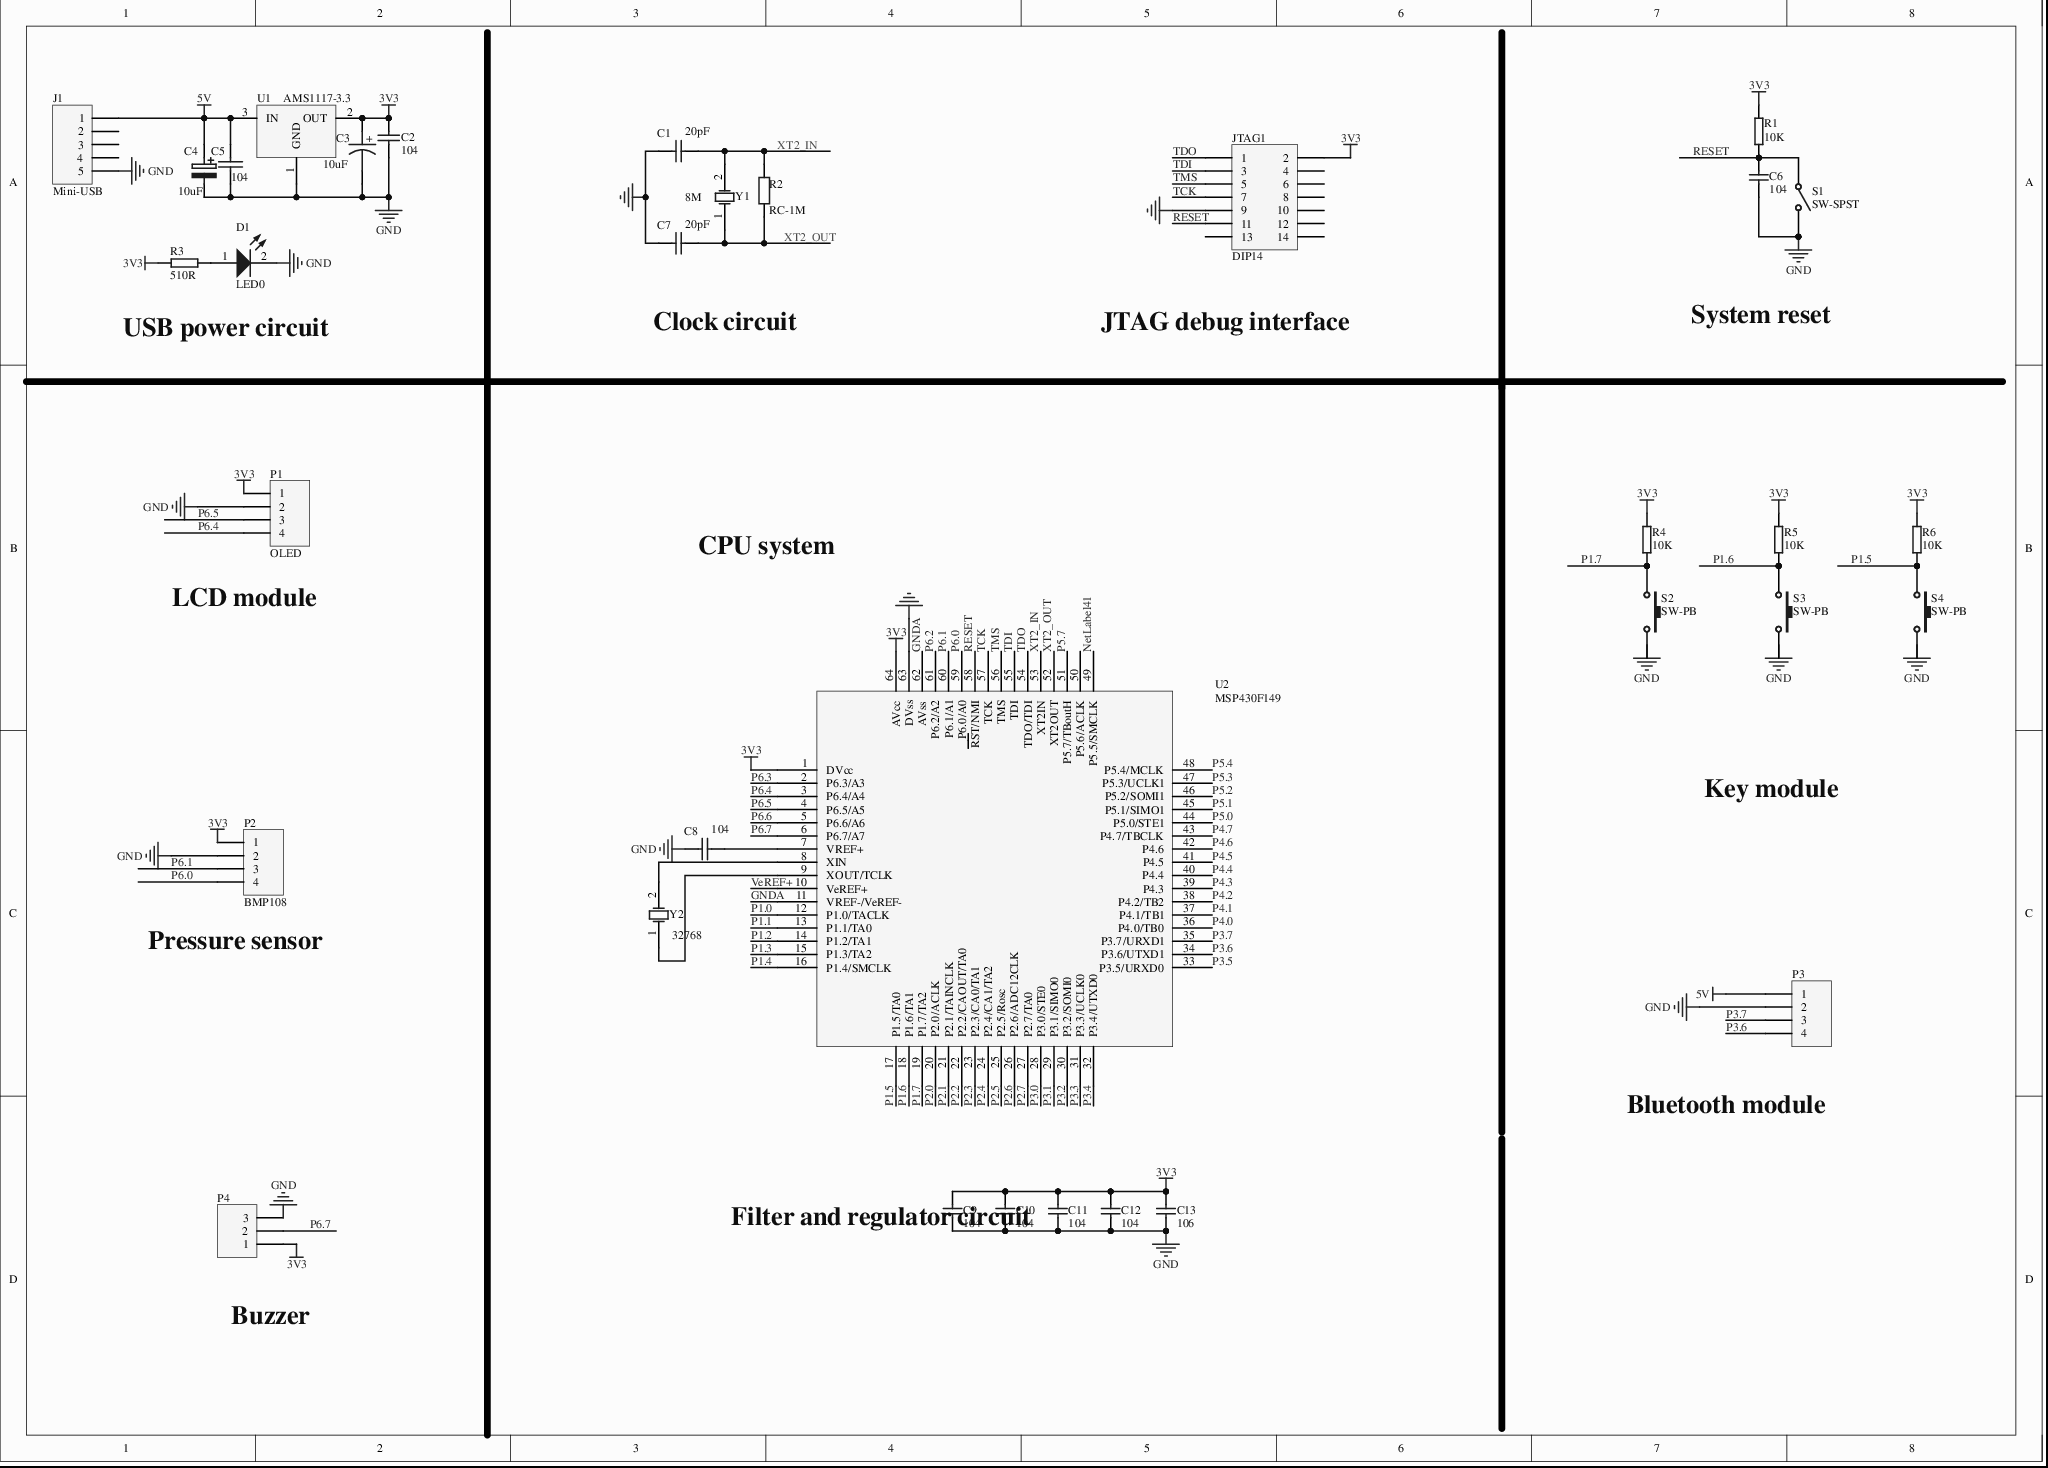
[diagram p0: MISC82806-6.SchDoc]
# Altium project MISC82806-6.PrjPcb
1 sheet, 34 parts. Net scope: global (net labels, ports and power ports of the same name join across sheets).
Board file: MISC82806.PcbDoc

## Sheet MISC82806-6.SchDoc
size A3

### Parts
C1  value 20pF  [0805C]  (hidden comment: S0805-20P)
C2  104  [0603C]
C3  10uF  [贴片电容]
C4  10uF  [0805C]
C5  104  [0603C]
C6  104  [0603C]
C7  value 20pF  [0805C]  (hidden comment: S0805-20P)
C8  value 104  [0805C]  (hidden comment: S0805-20P)
C9  104  [0603C]
C10  104  [0603C]
C11  104  [0603C]
C12  104  [0603C]
C13  106  [0805C]
D1  LED0  [LED0603-RD]
J1  Mini-USB  [USB-MINI-A]
JTAG1  DIP14  [HDR2X7]
P1  OLED  [HDR1X4H]
P2  BMP108  [HDR1X4H]
P3  Bluetooth module  [HDR1X4]  (value not drawn)
P4  Buzzer  [HDR1X3]  (value not drawn)
R1  10K  [0603R]
R2  RC-1M  [0805R]
R3  510R  [0603R]
R4  10K  [0603R]
R5  10K  [0603R]
R6  10K  [0603R]
S1  SW-SPST  [SPST-2]
S2  SW-PB  [SPST-2]
S3  SW-PB  [SPST-2]
S4  SW-PB  [SPST-2]
U1  AMS1117-3.3  [AMS1117-3.3]
U2  MSP430F149  [MSP430F149]
Y1  8M  [XTAL-SMD-NX3215SA-32.768K-STD-MUS-2]
Y2  32768  [XTAL-SMD-NX3215SA-32.768K-STD-MUS-2]

### Nets
3V3: C2.1 C3.1 C9.1 C10.1 C11.1 C12.1 C13.1 JTAG1.2 P1.1 P2.1 P4.1 R1.2 R3.2 R4.2 R5.2 R6.2 U1.2(OUT) U2.1(DVcc) U2.64(AVcc)
5V: C4.1 C5.1 J1.1 P3.1 U1.3(IN)
GND: C1.1 C2.2 C3.2 C4.2 C5.2 C6.2 C7.1 C8.1 C9.2 C10.2 C11.2 C12.2 C13.2 D1.2(K) J1.5 JTAG1.9 P1.2 P2.2 P3.2 P4.3 S1.2(NO) U1.1(GND) U2.63(DVss)
GNDA: U2.11(VREF-/VeREF-) U2.62(AVss)
NetLabel41: U2.49(P5.5/SMCLK)
P1.0: U2.12(P1.0/TACLK)
P1.1: U2.13(P1.1/TA0)
P1.2: U2.14(P1.2/TA1)
P1.3: U2.15(P1.3/TA2)
P1.4: U2.16(P1.4/SMCLK)
P1.5: R6.1 S4.1 U2.17(P1.5/TA0)
P1.6: R5.1 S3.1 U2.18(P1.6/TA1)
P1.7: R4.1 S2.1 U2.19(P1.7/TA2)
P2.0: U2.20(P2.0/ACLK)
P2.1: U2.21(P2.1/TAINCLK)
P2.2: U2.22(P2.2/CAOUT/TA0)
P2.3: U2.23(P2.3/CA0/TA1)
P2.4: U2.24(P2.4/CA1/TA2)
P2.5: U2.25(P2.5/Rosc)
P2.6: U2.26(P2.6/ADC12CLK)
P2.7: U2.27(P2.7/TA0)
P3.0: U2.28(P3.0/STE0)
P3.1: U2.29(P3.1/SIMO0)
P3.2: U2.30(P3.2/SOMI0)
P3.3: U2.31(P3.3/UCLK0)
P3.4: U2.32(P3.4/UTXD0)
P3.5: U2.33(P3.5/URXD0)
P3.6: P3.4 U2.34(P3.6/UTXD1)
P3.7: P3.3 U2.35(P3.7/URXD1)
P4.0: U2.36(P4.0/TB0)
P4.1: U2.37(P4.1/TB1)
P4.2: U2.38(P4.2/TB2)
P4.3: U2.39(P4.3)
P4.4: U2.40(P4.4)
P4.5: U2.41(P4.5)
P4.6: U2.42(P4.6)
P4.7: U2.43(P4.7/TBCLK)
P5.0: U2.44(P5.0/STE1)
P5.1: U2.45(P5.1/SIMO1)
P5.2: U2.46(P5.2/SOMI1)
P5.3: U2.47(P5.3/UCLK1)
P5.4: U2.48(P5.4/MCLK)
P5.7: U2.51(P5.7/TBoutH)
P6.0: P2.4 U2.59(P6.0/A0)
P6.1: P2.3 U2.60(P6.1/A1)
P6.2: U2.61(P6.2/A2)
P6.3: U2.2(P6.3/A3)
P6.4: P1.4 U2.3(P6.4/A4)
P6.5: P1.3 U2.4(P6.5/A5)
P6.6: U2.5(P6.6/A6)
P6.7: P4.2 U2.6(P6.7/A7)
RESET: C6.1 JTAG1.11 R1.1 S1.1(COMMON) U2.58(~{RS}T/NMI)
TCK: JTAG1.7 U2.57(TCK)
TDI: JTAG1.3 U2.55(TDI)
TDO: JTAG1.1 U2.54(TDO/TDI)
TMS: JTAG1.5 U2.56(TMS)
VeREF+: U2.10(VeREF+)
XT2_IN: C1.2 R2.2 U2.53(XT2IN) Y1.2(OSC2)
XT2_OUT: C7.2 R2.1 U2.52(XT2OUT) Y1.1(OSC1)
NetC8_2: C8.2 U2.7(VREF+)
NetD1_1: D1.1(A) R3.1
NetU2_8: U2.8(XIN) Y2.2(OSC2)
NetU2_9: U2.9(XOUT/TCLK) Y2.1(OSC1)

Not connected (* = marked no-connect by the designer): J1 2 3 4; JTAG1 4 6 8 10 12 13 14; S2 2; S3 2; S4 2; U2 50(P5.6/ACLK)

### Notes on the sheet
- USB power circuit
- Clock circuit
- JTAG debug interface
- System reset
- CPU system
- (near P1) LCD module
- Key module
- (near P2) Pressure sensor
- Bluetooth module
- Filter and regulator circuit
- Buzzer
- STM32F103C8T6
- Labels drawn without touching a wire or pin: GND

### Library data of the parts
C1 C2 C7 C8 = Cap: Capacitor; Published: 8-Jun-2000; LatestRevisionDate: 17-Jul-2002; LatestRevisionNote: Re-released for DXP Platform.; Publisher: Altium Limited
  C2: PackageReference: RAD-0.3
C3 = CAPACITOR POL: Capacitor
C4 = ELECTRO2
C5 = CAP: Capacitor
C6 C9-C13 = CAP1: Capacitor; Tolerate: 50V; Value: 100nF; TOL: 10%; ERP: 0103020075; PCB_Layout: Top Layer SMC; Revision: 2012-3-28; Publisher: ZL_A0OFFICE
D1 = LED0: Typical INFRARED GaAs LED
J1 = Header 5: Header, 5-Pin
JTAG1 = DIP14: Connectors; Set Position: 0.5; Published: 8-Jun-2000; LatestRevisionDate: 17-Jul-2002; LatestRevisionNote: Re-released for DXP Platform.; PackageReference: AXIAL-0.6; Publisher: Altium Limited
P1 P2 = Header 4H: Header, 4-Pin, Right Angle; LatestRevisionDate: 17-Jul-2002; LatestRevisionNote: Re-released for DXP Platform.; Publisher: Altium Limited
P3 = Header 4: Header, 4-Pin; LatestRevisionDate: 17-Jul-2002; LatestRevisionNote: Re-released for DXP Platform.; Publisher: Altium Limited
P4 = Header 3: Header, 3-Pin; LatestRevisionDate: 17-Jul-2002; LatestRevisionNote: Re-released for DXP Platform.; Publisher: Altium Limited
R1 R3-R6 = R
R2 = Res2: Resistor; Published: 8-Jun-2000; LatestRevisionDate: 17-Jul-2002; LatestRevisionNote: Re-released for DXP Platform.; Value: RC-1M; Publisher: Altium Limited
S1 = SW-SPST: Single-Pole, Single-Throw Switch
S2-S4 = SW-PB: Switch; Published: 24-Mar-1999; LatestRevisionDate: 17-Jul-2002; LatestRevisionNote: Re-released for DXP Platform.; PackageReference: SPST-2; PackageDescription: Switch; 2 Leads; Publisher: Altium Limited
U1 = LT1085CM-3.3
U2 = MSP430F149: MCU
Y1 Y2 = XTAL: Crystal Oscillator; Published: *; LatestRevisionDate: *; LatestRevisionNote: *; Publisher: *